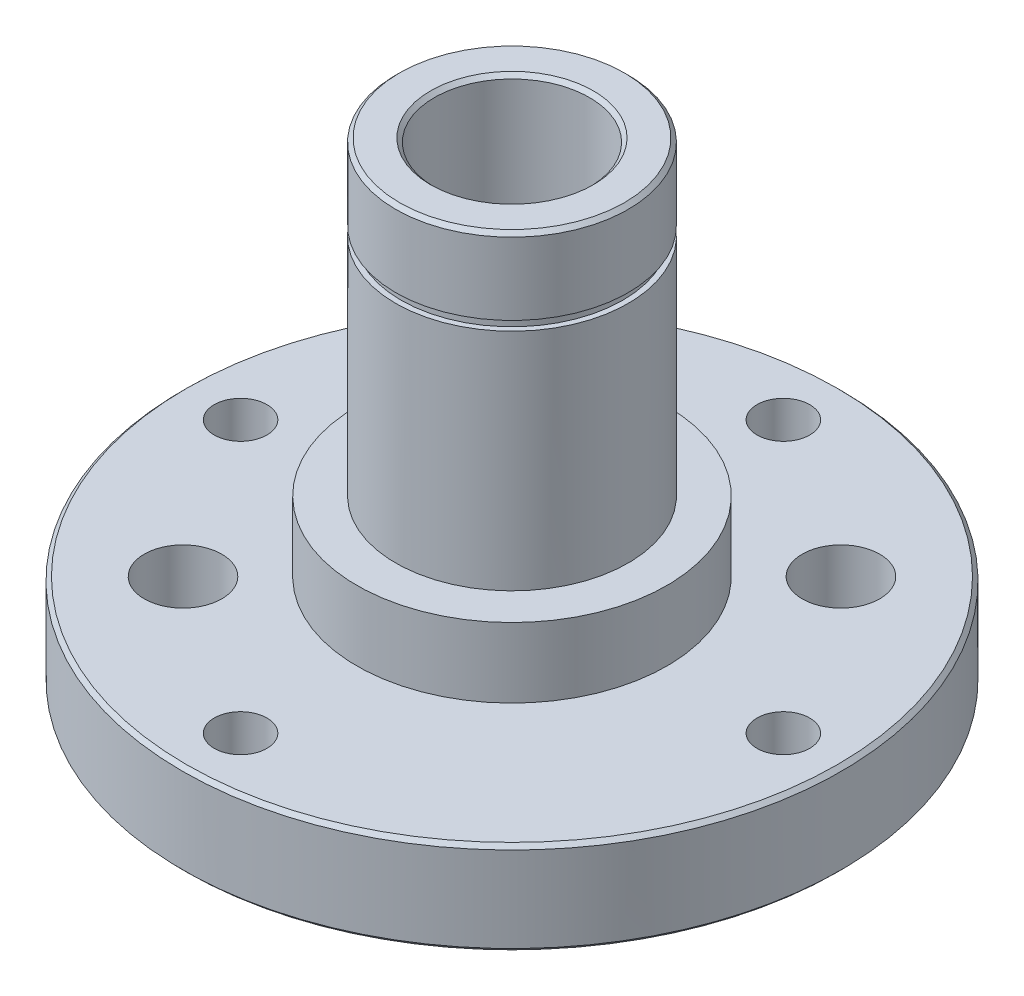
SolidWorks part; units mm, degrees
ref_plane "Front Plane" through (0, 0, 0) normal (0, 0, 1) x (1, 0, 0)
ref_plane "Top Plane" through (0, 0, 0) normal (0, 1, 0) x (1, 0, 0)
ref_plane "Right Plane" through (0, 0, 0) normal (1, 0, 0) x (0, 0, -1)
sketch "Sketch1" plane through (0, 0, 0) normal (0, 0, 1) x (1, 0, 0)
  line L0 (0, 0) -> (0, 25741.0304) construction
  line L1 (0, 0) -> (42.5, 0)
  line L2 (42.5, 0) -> (42.5, 12)
  line L3 (42.5, 12) -> (20, 12)
  line L4 (20, 12) -> (20, 21)
  line L5 (20, 21) -> (15, 21)
  line L6 (15, 61) -> (0, 61)
  line L7 (15, 61) -> (15, 21)
  line L8 (0, 61) -> (0, 0)
  dimension "D1" = 85
  dimension "D2" = 40
  dimension "D3" = 30
  dimension "D4" = 12
  dimension "D5" = 9
  dimension "D6" = 61
revolve "Revolve1" add sketch "Sketch1" angle 360 about L0
sketch "Sketch2" plane through (0, 61, 0) normal (0, 1, 0) x (1, 0, 0)
  circle A0 centre (0, 0) radius 10
  dimension "D1" = 20
extrude "Cut-Extrude1" cut sketch "Sketch2" against normal through all
sketch "Sketch3" plane through (0, 0, 0) normal (0, 0, 1) x (1, 0, 0)
  line L0 (15, 21) -> (15, 61) construction
  line L1 (15, 51.2) -> (14.3, 51.2)
  line L2 (15, 51.2) -> (15, 50)
  line L3 (15, 50) -> (14.3, 50)
  line L4 (14.3, 51.2) -> (14.3, 50)
  line L5 (15, 61) -> (-15, 61) construction
  dimension "D1" = 14.3
  dimension "D2" = 9.8
  dimension "D3" = 1.2
revolve "Cut-Revolve1" cut sketch "Sketch3" angle 360 about axis through (0, 0, 0) along (0, -1, 0)
hole_wizard "M8 Tapped Hole1" positions "Sketch4" profile "Sketch5" tap size "M8" standard "GB" end condition through all
sketch "Sketch4" plane through (0, 12, 0) normal (0, 1, 0) x (1, 0, 0)
  circle A0 centre (0, 0) radius 35 construction
  point P0 (35, 0)
  point P13 (0, -35)
  point P14 (-35, 0)
  point P15 (0, 35)
  point P16 (0, 0)
  dimension "D1" = 70
  dimension "D2" = 4
sketch "Sketch5" plane through (35, 12, 0) normal (1, 0, 0) x (0, 0, 1)
  line L0 (0, 0) -> (0, 12)
  line L1 (0, 12) -> (3.4, 12)
  line L2 (3.4, 12) -> (3.4, 0)
  line L5 (3.4, 0) -> (0, 0)
  line L11 (0, -6.35) -> (0, 107.95) construction
  dimension "通孔螺纹孔钻头直径" = 6.8
  dimension "通孔螺纹孔钻头深度" = 12
cosmetic thread "Cosmetic thread 1" parameters "D2"=8
cosmetic thread "Cosmetic thread 2" parameters "D2"=8
cosmetic thread "Cosmetic thread 3" parameters "D2"=8
cosmetic thread "Cosmetic thread 4" parameters "D2"=8
hole_wizard "Ø10.0 (10) Diameter Hole1" positions "Sketch6" profile "Sketch7" hole size "Ø10.0" standard "GB" end condition through all
sketch "Sketch6" plane through (0, 12, 0) normal (0, 1, 0) x (1, 0, 0)
  line L0 (0, 0) -> (-21.2132, -21.2132) construction
  line L2 (0, 0) -> (0, -35) construction
  circle A0 centre (0, 0) radius 30 construction
  point P0 (-21.2132, -21.2132)
  point P16 (21.2132, 21.2132)
  dimension "D1" = 60
  dimension "D2" = 45
sketch "Sketch7" plane through (-21.2132, 12, 21.2132) normal (1, 0, 0) x (0, 0, 1)
  line L0 (0, 0) -> (0, 12)
  line L1 (0, 12) -> (5, 12)
  line L2 (5, 12) -> (5, 0)
  line L5 (5, 0) -> (0, 0)
  line L11 (0, -6.35) -> (0, 107.95) construction
  dimension "通孔孔直径" = 10
  dimension "通孔孔深度" = 12
chamfer "Chamfer1" distance 0.5 angle 45 4 edges at (0, 0, -42.5) (0, 12, -42.5) (0, 61, -15) (0, 61, 10)
